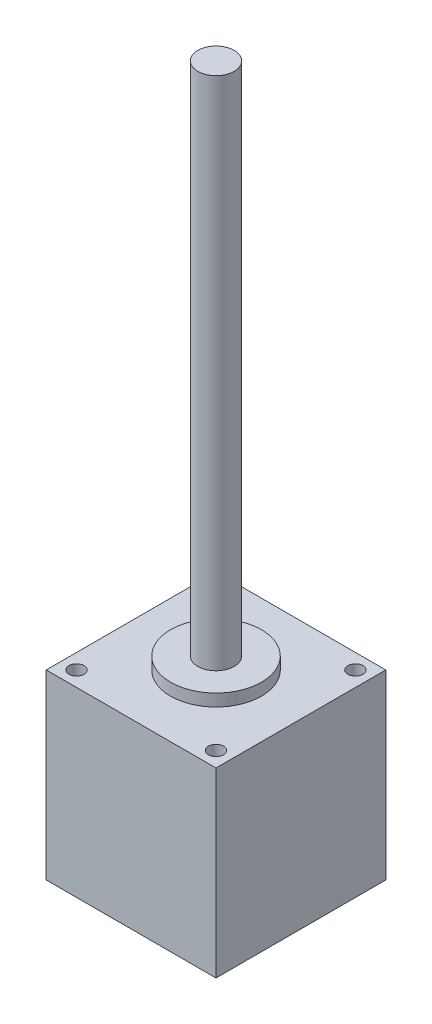
from build123d import *

# Parameters (mm, degrees)
SKETCH1_W             = 28
SKETCH1_H             = 28
BOSS_EXTRUDE1_DEPTH   = 30
SKETCH2_R             = 7.5
BOSS_EXTRUDE2_DEPTH   = 2
SKETCH3_R             = 3
BOSS_EXTRUDE3_DEPTH   = 85
SKETCH4_R             = 1
CUT_EXTRUDE1_DEPTH    = 3
M3_TAPPED_HOLE1_D     = 2.5
M3_TAPPED_HOLE1_DEPTH = 7.5
M3_TAPPED_HOLE1_TIP   = 0.751075774


with BuildPart() as part:
    # Sketch1 → Boss-Extrude1 (new body)
    with BuildSketch(Plane(origin=(0, 0, 0), x_dir=(1, 0, 0), z_dir=(0, 1, 0))):
        Rectangle(SKETCH1_W, SKETCH1_H)
    extrude(amount=BOSS_EXTRUDE1_DEPTH)

    # Sketch2 → Boss-Extrude2 (add)
    with BuildSketch(Plane(origin=(0, 30, 0), x_dir=(1, 0, 0), z_dir=(0, 1, 0))):
        with Locations(Location((0, 0, 0), (0, 0, 270))):
            Circle(SKETCH2_R)
    extrude(amount=BOSS_EXTRUDE2_DEPTH)

    # Sketch3 → Boss-Extrude3 (add)
    with BuildSketch(Plane(origin=(0, 32, 0), x_dir=(1, 0, 0), z_dir=(0, 1, 0))):
        with Locations(Location((0, 0, 0), (0, 0, 270))):
            Circle(SKETCH3_R)
    extrude(amount=BOSS_EXTRUDE3_DEPTH)

    # Sketch4 → Cut-Extrude1 (cut)
    with BuildSketch(Plane(origin=(0, 30, 0), x_dir=(1, 0, 0), z_dir=(0, 1, 0))):
        with Locations(Location((-11.5, -11.5, 0), (0, 0, 270))):
            Circle(SKETCH4_R)
        with Locations(Location((11.5, -11.5, 0), (0, 0, 270))):
            Circle(SKETCH4_R)
        with Locations(Location((-11.5, 11.5, 0), (0, 0, 270))):
            Circle(SKETCH4_R)
        with Locations(Location((11.5, 11.5, 0), (0, 0, 270))):
            Circle(SKETCH4_R)
    extrude(amount=-CUT_EXTRUDE1_DEPTH, mode=Mode.SUBTRACT)

    # M3 Tapped Hole1
    with Locations(Plane(origin=(0, 30, 0), x_dir=(1, 0, 0), z_dir=(0, 1, 0))):
        with Locations((-11.5, -11.5), (11.5, -11.5), (-11.5, 11.5), (11.5, 11.5)):
            Hole(M3_TAPPED_HOLE1_D / 2, depth=M3_TAPPED_HOLE1_DEPTH)
            with Locations((0, 0, -(M3_TAPPED_HOLE1_DEPTH + M3_TAPPED_HOLE1_TIP / 2))):  # 118° drill point
                Cone(0, M3_TAPPED_HOLE1_D / 2, M3_TAPPED_HOLE1_TIP, mode=Mode.SUBTRACT)


solid = part.part
